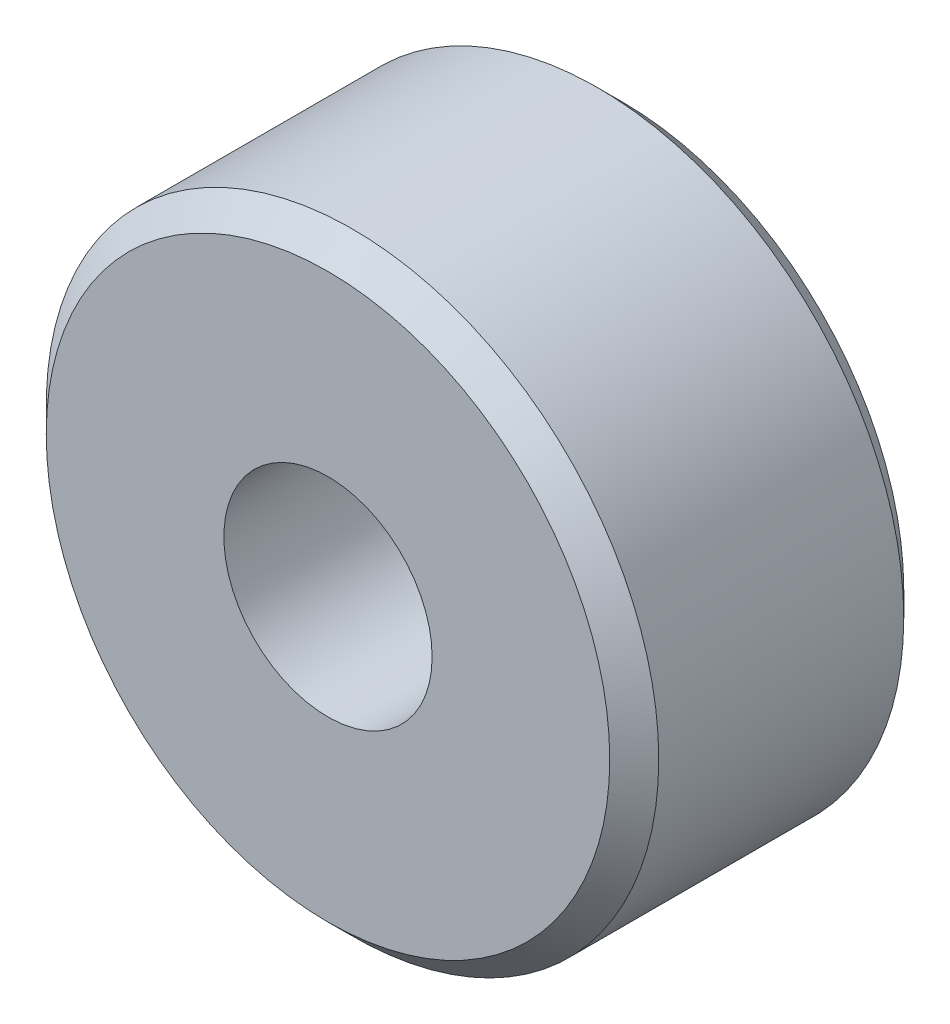
from build123d import *

# Parameters (mm, degrees)
SKETCH1_R           = 12.5
BOSS_EXTRUDE1_DEPTH = 12
M10_TAPPED_HOLE1_D  = 8.5
CHAMFER1_SIZE       = 1


with BuildPart() as part:
    # Sketch1 → Boss-Extrude1 (new body)
    with BuildSketch(Plane.XY):
        Circle(SKETCH1_R)
    extrude(amount=BOSS_EXTRUDE1_DEPTH)

    # M10 Tapped Hole1 (through all)
    with Locations(Plane.XY.offset(12)):
        with Locations((0, 0)):
            Hole(M10_TAPPED_HOLE1_D / 2)

    # Chamfer1
    chamfer1_edges = [part.edges().sort_by_distance(p)[0] for p in [
        (-12.5, 0, 0),
        (-12.5, 0, 12),
    ]]
    chamfer(chamfer1_edges, length=CHAMFER1_SIZE)


solid = part.part
